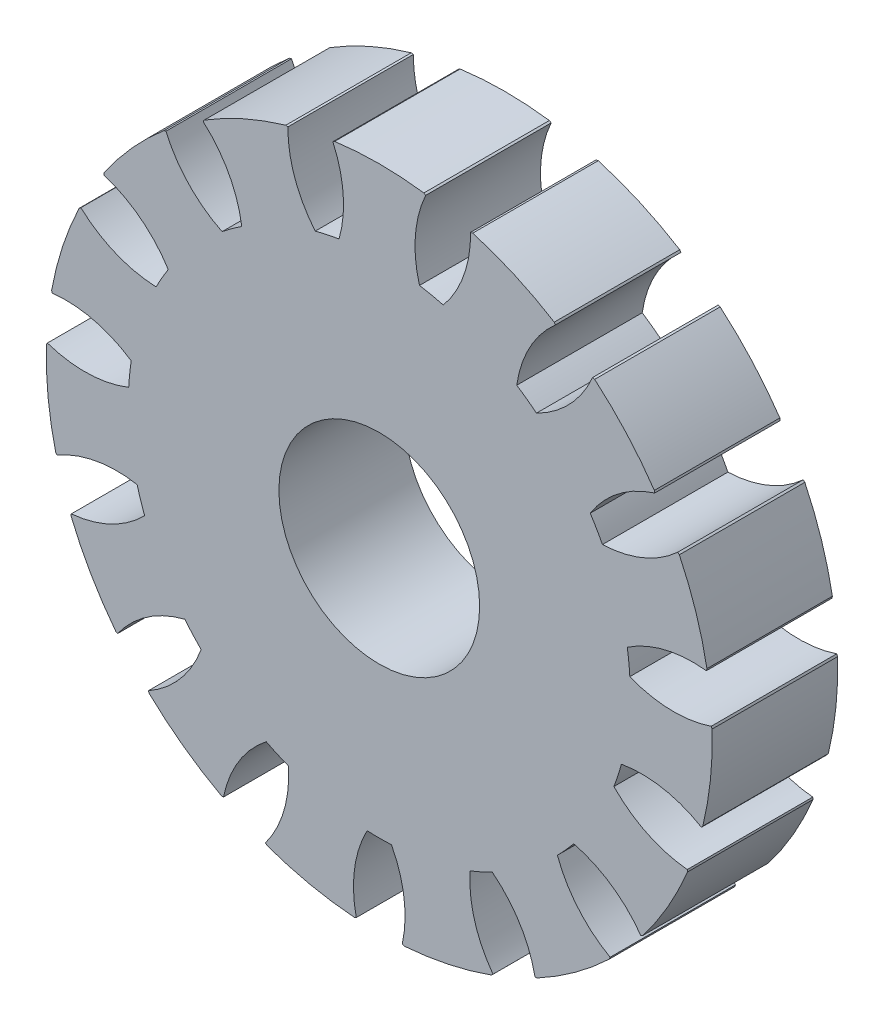
SolidWorks part; units mm, degrees
ref_plane "Front Plane" through (0, 0, 0) normal (0, 0, 1) x (1, 0, 0)
ref_plane "Top Plane" through (0, 0, 0) normal (0, 1, 0) x (1, 0, 0)
ref_plane "Right Plane" through (0, 0, 0) normal (1, 0, 0) x (0, 0, -1)
other "Configuration Table"
sketch "Sketch1" plane through (0, 0, 0) normal (0, 0, 1) x (1, 0, 0)
  circle A0 centre (0, 0) radius 10
  dimension "D1" = 20
extrude "Boss-Extrude1" add sketch "Sketch1" along normal blind 5
sketch "Sketch2" plane through (0, 0, 0) normal (0, 0, -1) x (-1, 0, 0)
  line L0 (0, 0) -> (0, 6.2508) construction
  circle A1 centre (0, 0) radius 10 construction
  arc A3 (-0.3745, 5.8479) -> (0.3745, 5.8479) centre (0, 4.9346) cw
  arc A4 (1.4709, 9.8912) -> (-1.4709, 9.8912) centre (0, 0) ccw
sketch "Sketch4" plane through (0, 0, 0) normal (0, 0, 1) x (1, 0, 0)
  line L0 (0, 0) -> (0, 6.2508) construction
  circle A0 centre (0, 0) radius 2.25
  dimension "D1" = 4.5
extrude "Cut-Extrude2" cut sketch "Sketch4" against normal mid plane 135
sketch "Sketch5" plane through (0, 0, 0) normal (0, 0, 1) x (1, 0, 0)
  line L1 (0, 1020) -> (0, 10) construction
  circle A0 centre (0, 0) radius 10 construction
  arc A1 (1.6021, 9.8708) -> (-1.6021, 9.8708) centre (0, 0) ccw
  arc A2 (-1.8497, 13.1038) -> (1.8497, 13.1038) centre (0, 10.3536) cw
  arc A3 (1.8497, 13.1038) -> (1.6021, 9.8708) centre (6.1089, 11.1516) ccw
  arc A4 (-1.8497, 13.1038) -> (-1.6021, 9.8708) centre (-6.1089, 11.1516) cw
  arc A5 (1.4709, 9.8912) -> (-1.4709, 9.8912) centre (0, 0) ccw construction
extrude "Boss-Extrude3" add sketch "Sketch5" along normal up to surface (5 mm away) up to face at (2.25, 0, 5)
pattern_circular "CirPattern2" count 15 over 360 about axis through (0, 0, 0) along (0, 0, 1) of "Boss-Extrude3"
sketch "Sketch3" plane through (0, 0, 0) normal (0, 0, -1) x (-1, 0, 0)
  circle A0 centre (0, 0) radius 2.25
  dimension "D1" = 4.5
sketch "Sketch6" plane through (0, 0, 0) normal (0, 0, 1) x (1, 0, 0)
  circle A0 centre (0, 0) radius 13.2703
extrude "Cut-Extrude3" cut sketch "Sketch6" along normal through all flip side to cut
sketch "Sketch7" plane through (0, 0, 5) normal (0, 0, 1) x (1, 0, 0)
  circle A0 centre (0, 0) radius 4
  dimension "D1" = 8
extrude "Cut-Extrude4" cut sketch "Sketch7" against normal through all
